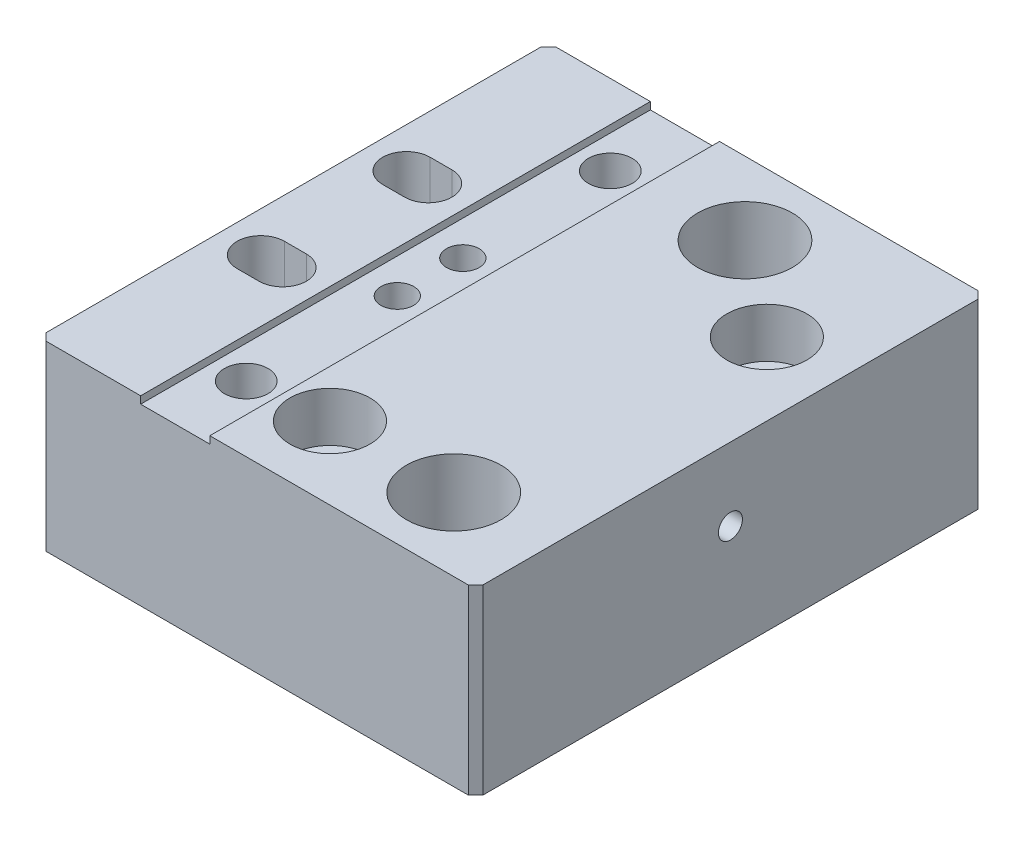
from build123d import *

# Parameters (mm, degrees)
SKETCH1_W                                            = 60
SKETCH1_H                                            = 25
BOSS_EXTRUDE1_DEPTH                                  = 35
SKETCH2_R                                            = 6.5
CUT_EXTRUDE1_DEPTH                                   = 53.440442409
SKETCH3_R                                            = 9
CUT_EXTRUDE2_DEPTH                                   = 10
SKETCH6_W                                            = 9.5
SKETCH6_H                                            = 70
CUT_EXTRUDE3_DEPTH                                   = 1
M4_TAPPED_HOLE1_D                                    = 3.3
M4_TAPPED_HOLE1_DEPTH                                = 12
M4_TAPPED_HOLE1_TIP                                  = 0.991420021
CUT_EXTRUDE4_DEPTH                                   = 7
M5_TAPPED_HOLE1_D                                    = 4.2
M5_TAPPED_HOLE1_DEPTH                                = 14
M5_TAPPED_HOLE1_TIP                                  = 1.2618073
HOLE_SIZE_PER_SOCKET_HEAD_CAP_SCREW_TYPE_D           = 4.5
HOLE_SIZE_PER_SOCKET_HEAD_CAP_SCREW_TYPE_CBORE_D     = 8
HOLE_SIZE_PER_SOCKET_HEAD_CAP_SCREW_TYPE_CBORE_DEPTH = 4
F_6_0_6_DIAMETER_HOLE2_D                             = 6
HOLE_SIZE_PER_SOCKET_HEAD_CAP_SCREW_2_D              = 6.6
HOLE_SIZE_PER_SOCKET_HEAD_CAP_SCREW_2_CBORE_D        = 11
HOLE_SIZE_PER_SOCKET_HEAD_CAP_SCREW_2_CBORE_DEPTH    = 6.8
M4_TAPPED_HOLE2_D                                    = 3.3
M4_TAPPED_HOLE2_DEPTH                                = 15
M4_TAPPED_HOLE2_TIP                                  = 0.991420021
CHAMFER1_SIZE                                        = 1


with BuildPart() as part:
    # Sketch1 → Boss-Extrude1 (new, symmetric)
    with BuildSketch(Plane.XY):
        with Locations((0, 12.5)):
            Rectangle(SKETCH1_W, SKETCH1_H)
    extrude(amount=BOSS_EXTRUDE1_DEPTH, both=True)

    # Sketch2 → Cut-Extrude1 (cut, through all)
    with BuildSketch(Plane(origin=(0, 25, 0), x_dir=(1, 0, 0), z_dir=(0, 1, 0))):
        with Locations(Location((7, 25, 0), (0, 0, 270))):
            Circle(SKETCH2_R)
        with Locations(Location((17, -25, 0), (0, 0, 270))):
            Circle(SKETCH2_R)
        with BuildLine():
            Line((-24.5, 13.25), (-21.5, 13.25))
            ThreePointArc((-21.5, 13.25), (-18.25, 10), (-21.5, 6.75))
            Line((-21.5, 6.75), (-24.5, 6.75))
            ThreePointArc((-24.5, 6.75), (-27.75, 10), (-24.5, 13.25))
        make_face()
        with BuildLine():
            Line((-24.5, -6.75), (-21.5, -6.75))
            ThreePointArc((-21.5, -6.75), (-18.25, -10), (-21.5, -13.25))
            Line((-21.5, -13.25), (-24.5, -13.25))
            ThreePointArc((-24.5, -13.25), (-27.75, -10), (-24.5, -6.75))
        make_face()
    extrude(amount=-CUT_EXTRUDE1_DEPTH, mode=Mode.SUBTRACT)

    # Sketch3 → Cut-Extrude2 (cut)
    with BuildSketch(Plane.XZ):
        with Locations(Location((17, 25, 0), (0, 0, 270))):
            Circle(SKETCH3_R)
        with Locations(Location((7, -25, 0), (0, 0, 270))):
            Circle(SKETCH3_R)
    extrude(amount=-CUT_EXTRUDE2_DEPTH, mode=Mode.SUBTRACT)

    # Sketch6 → Cut-Extrude3 (cut)
    with BuildSketch(Plane(origin=(0, 25, 0), x_dir=(-1, 0, 0), z_dir=(0, 1, 0))):
        with Locations((11.25, 0)):
            Rectangle(SKETCH6_W, SKETCH6_H)
    extrude(amount=-CUT_EXTRUDE3_DEPTH, mode=Mode.SUBTRACT)

    # M4 Tapped Hole1
    with Locations(Plane(origin=(0, 24, 0), x_dir=(-1, 0, 0), z_dir=(0, 1, 0))):
        with Locations((11.25, 4.5), (11.25, -4.5)):
            Hole(M4_TAPPED_HOLE1_D / 2, depth=M4_TAPPED_HOLE1_DEPTH)
            with Locations((0, 0, -(M4_TAPPED_HOLE1_DEPTH + M4_TAPPED_HOLE1_TIP / 2))):  # 118° drill point
                Cone(0, M4_TAPPED_HOLE1_D / 2, M4_TAPPED_HOLE1_TIP, mode=Mode.SUBTRACT)

    # Sketch10 → Cut-Extrude4 (cut)
    with BuildSketch(Plane.XZ):
        with BuildLine():
            Line((-21.5, -16), (-30, -16))
            ThreePointArc((-30, -16), (-36, -10), (-30, -4))
            Line((-30, -4), (-21.5, -4))
            ThreePointArc((-21.5, -4), (-15.5, -10), (-21.5, -16))
        make_face()
        with BuildLine():
            Line((-21.5, 4), (-30, 4))
            ThreePointArc((-30, 4), (-36, 10), (-30, 16))
            Line((-30, 16), (-21.5, 16))
            ThreePointArc((-21.5, 16), (-15.5, 10), (-21.5, 4))
        make_face()
    extrude(amount=-CUT_EXTRUDE4_DEPTH, mode=Mode.SUBTRACT)

    # M5 Tapped Hole1
    with Locations(Plane(origin=(0, 0, -35), x_dir=(-1, 0, 0), z_dir=(0, 0, -1))):
        with Locations((-22.5, 19), (-22.5, 6), (22.5, 19), (22.5, 6)):
            Hole(M5_TAPPED_HOLE1_D / 2, depth=M5_TAPPED_HOLE1_DEPTH)
            with Locations((0, 0, -(M5_TAPPED_HOLE1_DEPTH + M5_TAPPED_HOLE1_TIP / 2))):  # 118° drill point
                Cone(0, M5_TAPPED_HOLE1_D / 2, M5_TAPPED_HOLE1_TIP, mode=Mode.SUBTRACT)

    # Hole size per socket head cap screw type (through all)
    with Locations(Plane.XZ):
        with Locations((-11.25, -4.5), (-11.25, 4.5)):
            CounterBoreHole(HOLE_SIZE_PER_SOCKET_HEAD_CAP_SCREW_TYPE_D / 2, HOLE_SIZE_PER_SOCKET_HEAD_CAP_SCREW_TYPE_CBORE_D / 2, HOLE_SIZE_PER_SOCKET_HEAD_CAP_SCREW_TYPE_CBORE_DEPTH)

    # Ø6.0 (6) Diameter Hole2 (through all)
    with Locations(Plane(origin=(0, 0, 0), x_dir=(-1, 0, 0), z_dir=(0, -1, 0))):
        with Locations((11.5, -25), (11.5, 25)):
            Hole(F_6_0_6_DIAMETER_HOLE2_D / 2)

    # Hole size per socket head cap screw  2 (through all)
    with Locations(Plane(origin=(0, 25, 0), x_dir=(1, 0, 0), z_dir=(0, 1, 0))):
        with Locations((0, -25), (20, 15)):
            CounterBoreHole(HOLE_SIZE_PER_SOCKET_HEAD_CAP_SCREW_2_D / 2, HOLE_SIZE_PER_SOCKET_HEAD_CAP_SCREW_2_CBORE_D / 2, HOLE_SIZE_PER_SOCKET_HEAD_CAP_SCREW_2_CBORE_DEPTH)

    # M4 Tapped Hole2
    with Locations(Plane(origin=(30, 0, 0), x_dir=(0, 0, -1), z_dir=(1, 0, 0))):
        with Locations((0, 15)):
            Hole(M4_TAPPED_HOLE2_D / 2, depth=M4_TAPPED_HOLE2_DEPTH)
            with Locations((0, 0, -(M4_TAPPED_HOLE2_DEPTH + M4_TAPPED_HOLE2_TIP / 2))):  # 118° drill point
                Cone(0, M4_TAPPED_HOLE2_D / 2, M4_TAPPED_HOLE2_TIP, mode=Mode.SUBTRACT)

    # Chamfer1
    chamfer1_edges = [part.edges().sort_by_distance(p)[0] for p in [
        (30, 12.5, 35),
        (-30, 12.5, 35),
        (30, 12.5, -35),
        (-30, 12.5, -35),
    ]]
    chamfer(chamfer1_edges, length=CHAMFER1_SIZE)


solid = part.part
